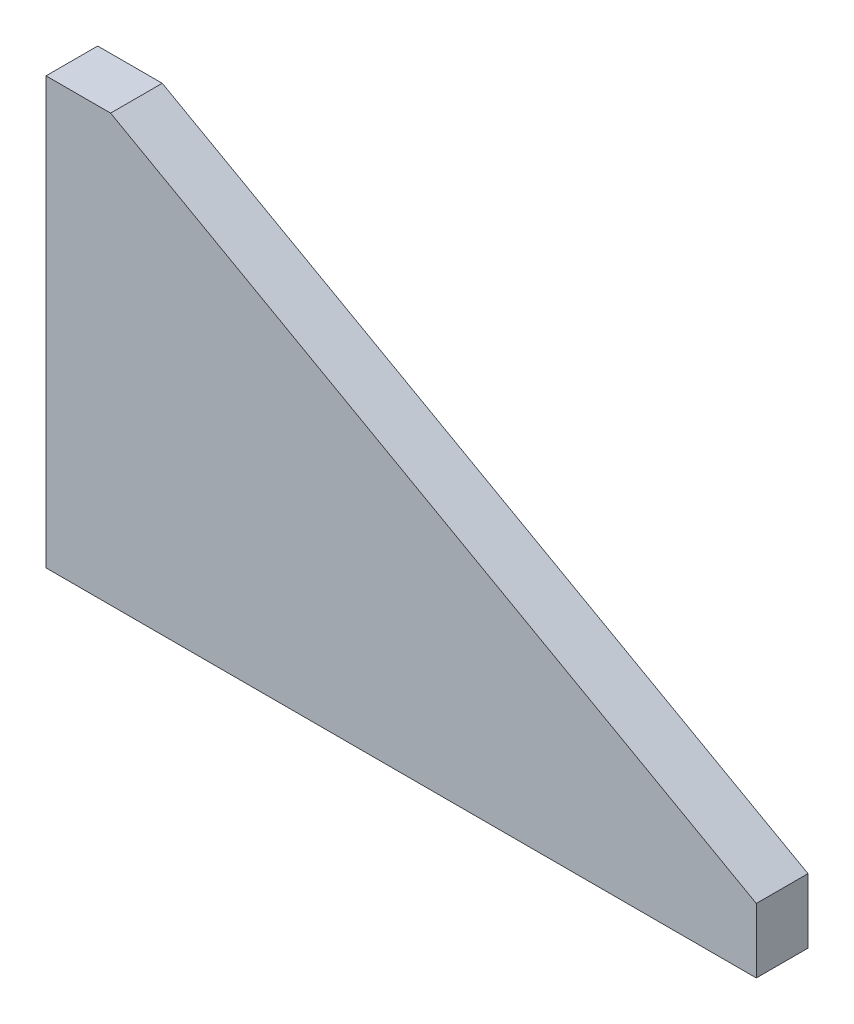
from build123d import *

# Parameters (mm, degrees)
BOSS_EXTRUDE1_DEPTH = 8


with BuildPart() as part:
    # Sketch1 → Boss-Extrude1 (new body)
    with BuildSketch(Plane.XY):
        Polygon((10, 66), (110, 10), (110, 0), (0, 0), (0, 66), align=None)
    extrude(amount=BOSS_EXTRUDE1_DEPTH)


solid = part.part
